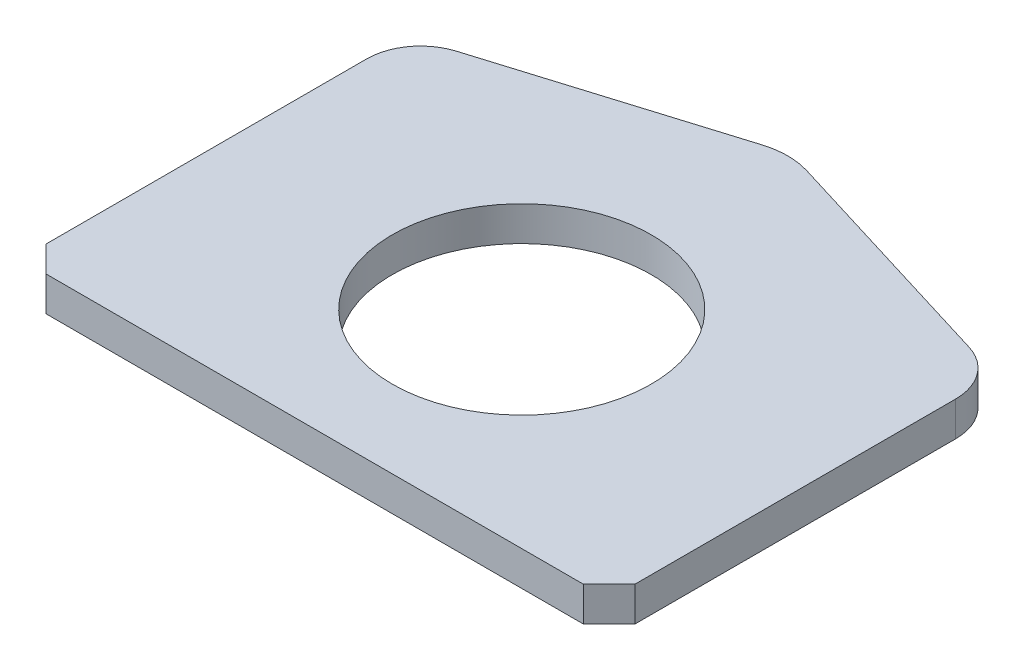
from build123d import *

# Parameters (mm, degrees)
SKETCH1_R           = 60
BOSS_EXTRUDE1_DEPTH = 16


with BuildPart() as part:
    # Sketch1 → Boss-Extrude1 (new body)
    with BuildSketch(Plane(origin=(0, 0, 0), x_dir=(1, 0, 0), z_dir=(0, 1, 0))):
        with BuildLine():
            Line((-124.5, 0), (124.5, 0))
            Line((124.5, 0), (136.5, 12))
            Line((136.5, 12), (136.5, 160.6))
            ThreePointArc((136.5, 160.6), (131.600675284, 175.464819311), (118.822971749, 184.503432489))
            Line((118.822971749, 184.503432489), (10.252160448, 217.764805485))
            ThreePointArc((10.252160448, 217.764805485), (0, 219.3), (-10.252160448, 217.764805485))
            Line((-10.252160448, 217.764805485), (-118.822971749, 184.503432489))
            ThreePointArc((-118.822971749, 184.503432489), (-131.600675284, 175.464819311), (-136.5, 160.6))
            Line((-136.5, 160.6), (-136.5, 12))
            Line((-136.5, 12), (-124.5, 0))
        make_face()
        with Locations(Location((0, 96, 0), (0, 0, 270))):
            Circle(SKETCH1_R, mode=Mode.SUBTRACT)
    extrude(amount=BOSS_EXTRUDE1_DEPTH)


solid = part.part
